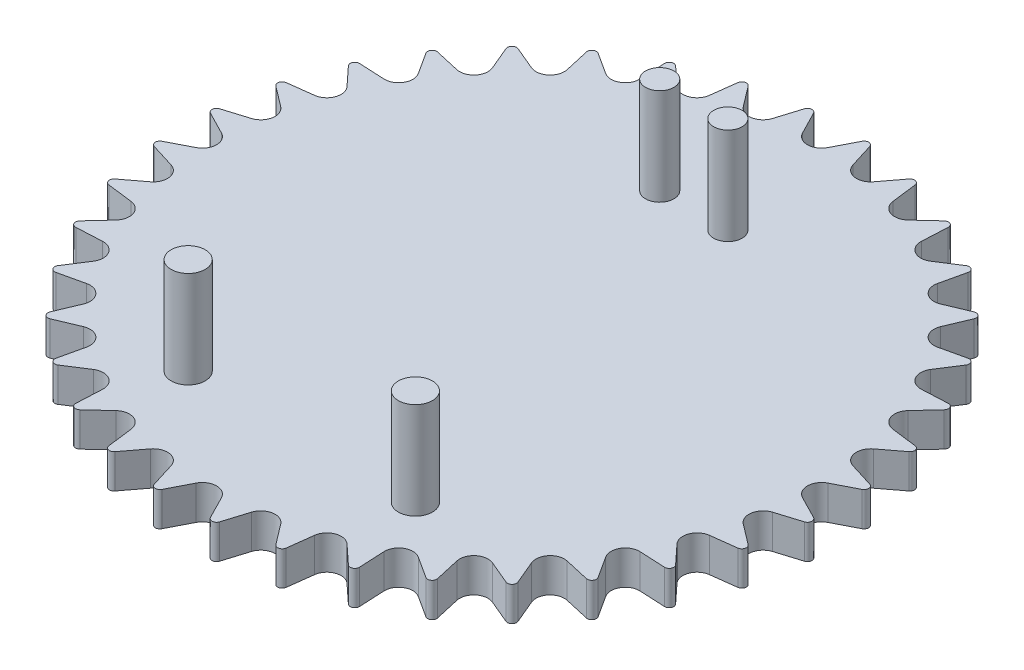
from build123d import *

# Parameters (mm, degrees)
SKETCH_1_R          = 290
EXTRUDE_1_DEPTH     = 30
SKETCH_2_R          = 12.5
SKETCH_2_R_2        = 15
EXTRUDE_2_DEPTH     = 85
SKETCH_4_R          = 330.934744746
CUT_EXTRUDE_1_DEPTH = 30
SKETCH_6_R          = 40
BOSS_EXTRUDE3_DEPTH = 50


with BuildPart() as part:
    # 草图1 → 凸台-拉伸1 (new body)
    with BuildSketch(Plane(origin=(0, 0, 0), x_dir=(1, 0, 0), z_dir=(0, 1, 0))):
        with Locations(Location((0, 0, 0), (0, 0, 270))):
            Circle(SKETCH_1_R)
    extrude(amount=EXTRUDE_1_DEPTH)

    # 草图2 → 凸台-拉伸2 (add)
    with BuildSketch(Plane(origin=(0, 30, 0), x_dir=(1, 0, 0), z_dir=(0, 1, 0))):
        with Locations(Location((-30, 160, 0), (0, 0, 270))):
            Circle(SKETCH_2_R)
        with Locations(Location((30, 160, 0), (0, 0, 270))):
            Circle(SKETCH_2_R)
        with Locations(Location((-100, -185, 0), (0, 0, 270))):
            Circle(SKETCH_2_R_2)
        with Locations(Location((100, -185, 0), (0, 0, 270))):
            Circle(SKETCH_2_R_2)
    extrude(amount=EXTRUDE_2_DEPTH)

    # 草图4 → 切除-拉伸1 (cut)
    with BuildSketch(Plane(origin=(0, 30, 0), x_dir=(1, 0, 0), z_dir=(0, 1, 0))):
        Circle(SKETCH_4_R)
        with BuildLine():
            Line((-21.368609629, 286.739555153), (-11.118539989, 266.787901567))
            ThreePointArc((-11.118539989, 266.787901567), (0, 260), (11.118539989, 266.787901567))
            Line((11.118539989, 266.787901567), (21.368609629, 286.739555153))
            ThreePointArc((21.368609629, 286.739555153), (22.993156883, 288.413400425), (25.275165397, 288.896462447))
            ThreePointArc((25.275165397, 288.896462447), (27.438622234, 288.024472603), (28.747828783, 286.093957131))
            Line((28.747828783, 286.093957131), (35.377608547, 264.66550808))
            ThreePointArc((35.377608547, 264.66550808), (45.148526193, 256.050015783), (57.276857314, 260.804079666))
            Line((57.276857314, 260.804079666), (70.835773651, 278.672716888))
            ThreePointArc((70.835773651, 278.672716888), (72.726300563, 280.03903302), (75.05752308, 280.118489624))
            ThreePointArc((75.05752308, 280.118489624), (77.036692699, 278.884066928), (77.990778965, 276.755538993))
            Line((77.990778965, 276.755538993), (80.79882635, 254.501387058))
            ThreePointArc((80.79882635, 254.501387058), (88.925237265, 244.320081404), (101.694846313, 246.895857777))
            Line((101.694846313, 246.895857777), (118.150628536, 262.138549136))
            ThreePointArc((118.150628536, 262.138549136), (120.249692402, 263.155821303), (122.559295905, 262.829258241))
            ThreePointArc((122.559295905, 262.829258241), (124.294042239, 261.269910001), (124.864018794, 259.008043847))
            Line((124.864018794, 259.008043847), (123.7650127, 236.604370174))
            ThreePointArc((123.7650127, 236.604370174), (130, 225.166604984), (143.022888867, 225.485830185))
            Line((143.022888867, 225.485830185), (161.875536359, 237.639434218))
            ThreePointArc((161.875536359, 237.639434218), (164.119358186, 238.276753118), (166.337166542, 237.554092844))
            ThreePointArc((166.337166542, 237.554092844), (167.774780201, 235.717199069), (167.943328596, 233.390720353))
            Line((167.943328596, 233.390720353), (162.970661767, 211.51824923))
            ThreePointArc((162.970661767, 211.51824923), (167.124778518, 199.171555211), (180.005253316, 197.224529744))
            Line((180.005253316, 197.224529744), (200.681937923, 205.919765341))
            ThreePointArc((200.681937923, 205.919765341), (203.002340321, 206.157766365), (205.060966544, 205.060966544))
            ThreePointArc((205.060966544, 205.060966544), (206.157766365, 203.002340321), (205.919765341, 200.681937923))
            Line((205.919765341, 200.681937923), (197.224529744, 180.005253316))
            ThreePointArc((197.224529744, 180.005253316), (199.171555211, 167.124778519), (211.51824923, 162.970661767))
            Line((211.51824923, 162.970661767), (233.390720353, 167.943328596))
            ThreePointArc((233.390720353, 167.943328596), (235.717199069, 167.774780201), (237.554092844, 166.337166542))
            ThreePointArc((237.554092844, 166.337166542), (238.276753118, 164.119358186), (237.639434218, 161.875536359))
            Line((237.639434218, 161.875536359), (225.485830185, 143.022888867))
            ThreePointArc((225.485830185, 143.022888867), (225.166604984, 130), (236.604370174, 123.7650127))
            Line((236.604370174, 123.7650127), (259.008043847, 124.864018794))
            ThreePointArc((259.008043847, 124.864018794), (261.269910001, 124.294042239), (262.829258241, 122.559295905))
            ThreePointArc((262.829258241, 122.559295905), (263.155821303, 120.249692402), (262.138549136, 118.150628536))
            Line((262.138549136, 118.150628536), (246.895857777, 101.694846313))
            ThreePointArc((246.895857777, 101.694846313), (244.320081404, 88.925237265), (254.501387058, 80.79882635))
            Line((254.501387058, 80.79882635), (276.755538993, 77.990778965))
            ThreePointArc((276.755538993, 77.990778965), (278.884066928, 77.036692699), (280.118489624, 75.05752308))
            ThreePointArc((280.118489624, 75.05752308), (280.03903302, 72.726300563), (278.672716888, 70.835773651))
            Line((278.672716888, 70.835773651), (260.804079666, 57.276857314))
            ThreePointArc((260.804079666, 57.276857314), (256.050015783, 45.148526193), (264.66550808, 35.377608547))
            Line((264.66550808, 35.377608547), (286.093957131, 28.747828783))
            ThreePointArc((286.093957131, 28.747828783), (288.024472603, 27.438622234), (288.896462447, 25.275165397))
            ThreePointArc((288.896462447, 25.275165397), (288.413400425, 22.993156883), (286.739555153, 21.368609629))
            Line((286.739555153, 21.368609629), (266.787901567, 11.118539989))
            ThreePointArc((266.787901567, 11.118539989), (260, 0), (266.787901567, -11.118539989))
            Line((266.787901567, -11.118539989), (286.739555153, -21.368609629))
            ThreePointArc((286.739555153, -21.368609629), (288.413400425, -22.993156883), (288.896462447, -25.275165397))
            ThreePointArc((288.896462447, -25.275165397), (288.024472603, -27.438622234), (286.093957131, -28.747828783))
            Line((286.093957131, -28.747828783), (264.66550808, -35.377608547))
            ThreePointArc((264.66550808, -35.377608547), (256.050015783, -45.148526193), (260.804079666, -57.276857314))
            Line((260.804079666, -57.276857314), (278.672716888, -70.835773651))
            ThreePointArc((278.672716888, -70.835773651), (280.03903302, -72.726300563), (280.118489624, -75.05752308))
            ThreePointArc((280.118489624, -75.05752308), (278.884066928, -77.036692699), (276.755538993, -77.990778965))
            Line((276.755538993, -77.990778965), (254.501387058, -80.79882635))
            ThreePointArc((254.501387058, -80.79882635), (244.320081404, -88.925237265), (246.895857777, -101.694846313))
            Line((246.895857777, -101.694846313), (262.138549136, -118.150628536))
            ThreePointArc((262.138549136, -118.150628536), (263.155821303, -120.249692402), (262.829258241, -122.559295905))
            ThreePointArc((262.829258241, -122.559295905), (261.269910001, -124.294042239), (259.008043847, -124.864018794))
            Line((259.008043847, -124.864018794), (236.604370174, -123.7650127))
            ThreePointArc((236.604370174, -123.7650127), (225.166604984, -130), (225.485830185, -143.022888867))
            Line((225.485830185, -143.022888867), (237.639434218, -161.875536359))
            ThreePointArc((237.639434218, -161.875536359), (238.276753118, -164.119358186), (237.554092844, -166.337166542))
            ThreePointArc((237.554092844, -166.337166542), (235.717199069, -167.774780201), (233.390720353, -167.943328596))
            Line((233.390720353, -167.943328596), (211.51824923, -162.970661767))
            ThreePointArc((211.51824923, -162.970661767), (199.171555211, -167.124778518), (197.224529744, -180.005253316))
            Line((197.224529744, -180.005253316), (205.919765341, -200.681937923))
            ThreePointArc((205.919765341, -200.681937923), (206.157766365, -203.002340321), (205.060966544, -205.060966544))
            ThreePointArc((205.060966544, -205.060966544), (203.002340321, -206.157766365), (200.681937923, -205.919765341))
            Line((200.681937923, -205.919765341), (180.005253316, -197.224529744))
            ThreePointArc((180.005253316, -197.224529744), (167.124778518, -199.171555211), (162.970661767, -211.51824923))
            Line((162.970661767, -211.51824923), (167.943328596, -233.390720353))
            ThreePointArc((167.943328596, -233.390720353), (167.774780201, -235.717199068), (166.337166542, -237.554092844))
            ThreePointArc((166.337166542, -237.554092844), (164.119358186, -238.276753118), (161.875536359, -237.639434218))
            Line((161.875536359, -237.639434218), (143.022888867, -225.485830185))
            ThreePointArc((143.022888867, -225.485830185), (130, -225.166604984), (123.7650127, -236.604370174))
            Line((123.7650127, -236.604370174), (124.864018794, -259.008043847))
            ThreePointArc((124.864018794, -259.008043847), (124.294042239, -261.269910001), (122.559295905, -262.829258241))
            ThreePointArc((122.559295905, -262.829258241), (120.249692402, -263.155821302), (118.150628536, -262.138549136))
            Line((118.150628536, -262.138549136), (101.694846313, -246.895857777))
            ThreePointArc((101.694846313, -246.895857777), (88.925237265, -244.320081404), (80.79882635, -254.501387058))
            Line((80.79882635, -254.501387058), (77.990778965, -276.755538993))
            ThreePointArc((77.990778965, -276.755538993), (77.036692699, -278.884066928), (75.05752308, -280.118489624))
            ThreePointArc((75.05752308, -280.118489624), (72.726300563, -280.03903302), (70.835773651, -278.672716888))
            Line((70.835773651, -278.672716888), (57.276857314, -260.804079665))
            ThreePointArc((57.276857314, -260.804079665), (45.148526193, -256.050015783), (35.377608547, -264.66550808))
            Line((35.377608547, -264.66550808), (28.747828783, -286.093957131))
            ThreePointArc((28.747828783, -286.093957131), (27.438622234, -288.024472603), (25.275165397, -288.896462447))
            ThreePointArc((25.275165397, -288.896462447), (22.993156883, -288.413400425), (21.368609629, -286.739555153))
            Line((21.368609629, -286.739555153), (11.118539989, -266.787901567))
            ThreePointArc((11.118539989, -266.787901567), (0, -260), (-11.118539989, -266.787901567))
            Line((-11.118539989, -266.787901567), (-21.368609629, -286.739555153))
            ThreePointArc((-21.368609629, -286.739555153), (-22.993156883, -288.413400425), (-25.275165397, -288.896462447))
            ThreePointArc((-25.275165397, -288.896462447), (-27.438622234, -288.024472603), (-28.747828783, -286.093957131))
            Line((-28.747828783, -286.093957131), (-35.377608547, -264.66550808))
            ThreePointArc((-35.377608547, -264.66550808), (-45.148526193, -256.050015783), (-57.276857314, -260.804079665))
            Line((-57.276857314, -260.804079665), (-70.835773651, -278.672716888))
            ThreePointArc((-70.835773651, -278.672716888), (-72.726300563, -280.03903302), (-75.05752308, -280.118489624))
            ThreePointArc((-75.05752308, -280.118489624), (-77.036692699, -278.884066928), (-77.990778965, -276.755538993))
            Line((-77.990778965, -276.755538993), (-80.79882635, -254.501387058))
            ThreePointArc((-80.79882635, -254.501387058), (-88.925237265, -244.320081404), (-101.694846313, -246.895857777))
            Line((-101.694846313, -246.895857777), (-118.150628536, -262.138549136))
            ThreePointArc((-118.150628536, -262.138549136), (-120.249692402, -263.155821302), (-122.559295905, -262.829258241))
            ThreePointArc((-122.559295905, -262.829258241), (-124.294042239, -261.269910001), (-124.864018794, -259.008043847))
            Line((-124.864018794, -259.008043847), (-123.7650127, -236.604370174))
            ThreePointArc((-123.7650127, -236.604370174), (-130, -225.166604984), (-143.022888867, -225.485830185))
            Line((-143.022888867, -225.485830185), (-161.875536359, -237.639434218))
            ThreePointArc((-161.875536359, -237.639434218), (-164.119358186, -238.276753118), (-166.337166542, -237.554092844))
            ThreePointArc((-166.337166542, -237.554092844), (-167.774780201, -235.717199068), (-167.943328596, -233.390720353))
            Line((-167.943328596, -233.390720353), (-162.970661767, -211.51824923))
            ThreePointArc((-162.970661767, -211.51824923), (-167.124778518, -199.171555211), (-180.005253316, -197.224529744))
            Line((-180.005253316, -197.224529744), (-200.681937923, -205.919765341))
            ThreePointArc((-200.681937923, -205.919765341), (-203.002340321, -206.157766365), (-205.060966544, -205.060966544))
            ThreePointArc((-205.060966544, -205.060966544), (-206.157766365, -203.002340321), (-205.919765341, -200.681937923))
            Line((-205.919765341, -200.681937923), (-197.224529744, -180.005253316))
            ThreePointArc((-197.224529744, -180.005253316), (-199.171555211, -167.124778518), (-211.51824923, -162.970661767))
            Line((-211.51824923, -162.970661767), (-233.390720353, -167.943328596))
            ThreePointArc((-233.390720353, -167.943328596), (-235.717199069, -167.774780201), (-237.554092844, -166.337166542))
            ThreePointArc((-237.554092844, -166.337166542), (-238.276753118, -164.119358186), (-237.639434218, -161.875536359))
            Line((-237.639434218, -161.875536359), (-225.485830185, -143.022888867))
            ThreePointArc((-225.485830185, -143.022888867), (-225.166604984, -130), (-236.604370174, -123.7650127))
            Line((-236.604370174, -123.7650127), (-259.008043847, -124.864018794))
            ThreePointArc((-259.008043847, -124.864018794), (-261.269910001, -124.294042239), (-262.829258241, -122.559295905))
            ThreePointArc((-262.829258241, -122.559295905), (-263.155821303, -120.249692402), (-262.138549136, -118.150628536))
            Line((-262.138549136, -118.150628536), (-246.895857777, -101.694846313))
            ThreePointArc((-246.895857777, -101.694846313), (-244.320081404, -88.925237265), (-254.501387058, -80.79882635))
            Line((-254.501387058, -80.79882635), (-276.755538993, -77.990778965))
            ThreePointArc((-276.755538993, -77.990778965), (-278.884066928, -77.036692699), (-280.118489624, -75.05752308))
            ThreePointArc((-280.118489624, -75.05752308), (-280.03903302, -72.726300563), (-278.672716888, -70.835773651))
            Line((-278.672716888, -70.835773651), (-260.804079666, -57.276857314))
            ThreePointArc((-260.804079666, -57.276857314), (-256.050015783, -45.148526193), (-264.66550808, -35.377608547))
            Line((-264.66550808, -35.377608547), (-286.093957131, -28.747828783))
            ThreePointArc((-286.093957131, -28.747828783), (-288.024472603, -27.438622234), (-288.896462447, -25.275165397))
            ThreePointArc((-288.896462447, -25.275165397), (-288.413400425, -22.993156883), (-286.739555153, -21.368609629))
            Line((-286.739555153, -21.368609629), (-266.787901567, -11.118539989))
            ThreePointArc((-266.787901567, -11.118539989), (-260, 0), (-266.787901567, 11.118539989))
            Line((-266.787901567, 11.118539989), (-286.739555153, 21.368609629))
            ThreePointArc((-286.739555153, 21.368609629), (-288.413400425, 22.993156883), (-288.896462447, 25.275165397))
            ThreePointArc((-288.896462447, 25.275165397), (-288.024472603, 27.438622234), (-286.093957131, 28.747828783))
            Line((-286.093957131, 28.747828783), (-264.66550808, 35.377608547))
            ThreePointArc((-264.66550808, 35.377608547), (-256.050015783, 45.148526193), (-260.804079666, 57.276857314))
            Line((-260.804079666, 57.276857314), (-278.672716888, 70.835773651))
            ThreePointArc((-278.672716888, 70.835773651), (-280.03903302, 72.726300563), (-280.118489624, 75.05752308))
            ThreePointArc((-280.118489624, 75.05752308), (-278.884066928, 77.036692699), (-276.755538993, 77.990778965))
            Line((-276.755538993, 77.990778965), (-254.501387058, 80.79882635))
            ThreePointArc((-254.501387058, 80.79882635), (-244.320081404, 88.925237265), (-246.895857777, 101.694846313))
            Line((-246.895857777, 101.694846313), (-262.138549136, 118.150628536))
            ThreePointArc((-262.138549136, 118.150628536), (-263.155821303, 120.249692402), (-262.829258241, 122.559295905))
            ThreePointArc((-262.829258241, 122.559295905), (-261.269910001, 124.294042239), (-259.008043847, 124.864018794))
            Line((-259.008043847, 124.864018794), (-236.604370174, 123.7650127))
            ThreePointArc((-236.604370174, 123.7650127), (-225.166604984, 130), (-225.485830185, 143.022888867))
            Line((-225.485830185, 143.022888867), (-237.639434218, 161.875536359))
            ThreePointArc((-237.639434218, 161.875536359), (-238.276753118, 164.119358186), (-237.554092844, 166.337166542))
            ThreePointArc((-237.554092844, 166.337166542), (-235.717199069, 167.774780201), (-233.390720353, 167.943328596))
            Line((-233.390720353, 167.943328596), (-211.51824923, 162.970661767))
            ThreePointArc((-211.51824923, 162.970661767), (-199.171555211, 167.124778519), (-197.224529744, 180.005253316))
            Line((-197.224529744, 180.005253316), (-205.919765341, 200.681937923))
            ThreePointArc((-205.919765341, 200.681937923), (-206.157766365, 203.002340321), (-205.060966544, 205.060966544))
            ThreePointArc((-205.060966544, 205.060966544), (-203.002340321, 206.157766365), (-200.681937923, 205.919765341))
            Line((-200.681937923, 205.919765341), (-180.005253316, 197.224529744))
            ThreePointArc((-180.005253316, 197.224529744), (-167.124778518, 199.171555211), (-162.970661767, 211.51824923))
            Line((-162.970661767, 211.51824923), (-167.943328596, 233.390720353))
            ThreePointArc((-167.943328596, 233.390720353), (-167.774780201, 235.717199069), (-166.337166542, 237.554092844))
            ThreePointArc((-166.337166542, 237.554092844), (-164.119358186, 238.276753118), (-161.875536359, 237.639434218))
            Line((-161.875536359, 237.639434218), (-143.022888867, 225.485830185))
            ThreePointArc((-143.022888867, 225.485830185), (-130, 225.166604984), (-123.7650127, 236.604370174))
            Line((-123.7650127, 236.604370174), (-124.864018794, 259.008043847))
            ThreePointArc((-124.864018794, 259.008043847), (-124.294042239, 261.269910001), (-122.559295905, 262.829258241))
            ThreePointArc((-122.559295905, 262.829258241), (-120.249692402, 263.155821303), (-118.150628536, 262.138549136))
            Line((-118.150628536, 262.138549136), (-101.694846313, 246.895857777))
            ThreePointArc((-101.694846313, 246.895857777), (-88.925237265, 244.320081404), (-80.79882635, 254.501387058))
            Line((-80.79882635, 254.501387058), (-77.990778965, 276.755538993))
            ThreePointArc((-77.990778965, 276.755538993), (-77.036692699, 278.884066928), (-75.05752308, 280.118489624))
            ThreePointArc((-75.05752308, 280.118489624), (-72.726300563, 280.03903302), (-70.835773651, 278.672716888))
            Line((-70.835773651, 278.672716888), (-57.276857314, 260.804079666))
            ThreePointArc((-57.276857314, 260.804079666), (-45.148526193, 256.050015783), (-35.377608547, 264.66550808))
            Line((-35.377608547, 264.66550808), (-28.747828783, 286.093957131))
            ThreePointArc((-28.747828783, 286.093957131), (-27.438622234, 288.024472603), (-25.275165397, 288.896462447))
            ThreePointArc((-25.275165397, 288.896462447), (-22.993156883, 288.413400425), (-21.368609629, 286.739555153))
        make_face(mode=Mode.SUBTRACT)
    extrude(amount=-CUT_EXTRUDE_1_DEPTH, mode=Mode.SUBTRACT)

    # 草图6 → Boss-Extrude3 (add)
    with BuildSketch(Plane.XZ):
        with Locations(Location((0, 0, 0), (0, 0, 90))):
            Circle(SKETCH_6_R)
    extrude(amount=BOSS_EXTRUDE3_DEPTH)


solid = part.part
